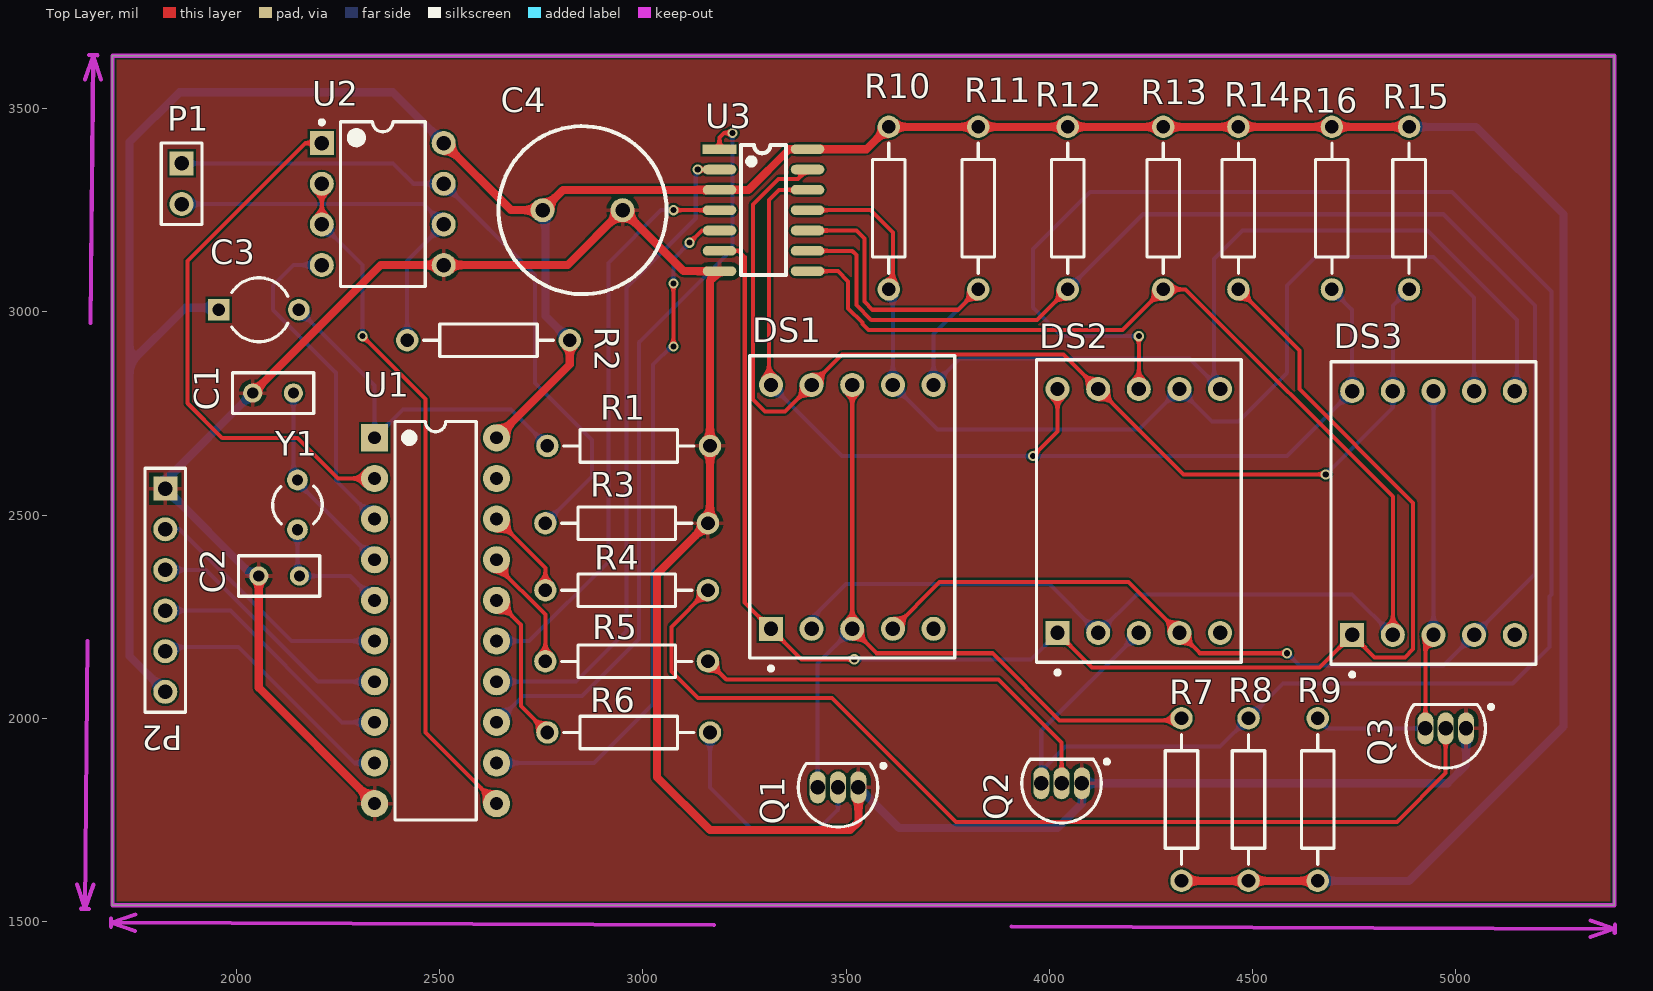
[diagram p0: Top Layer view]
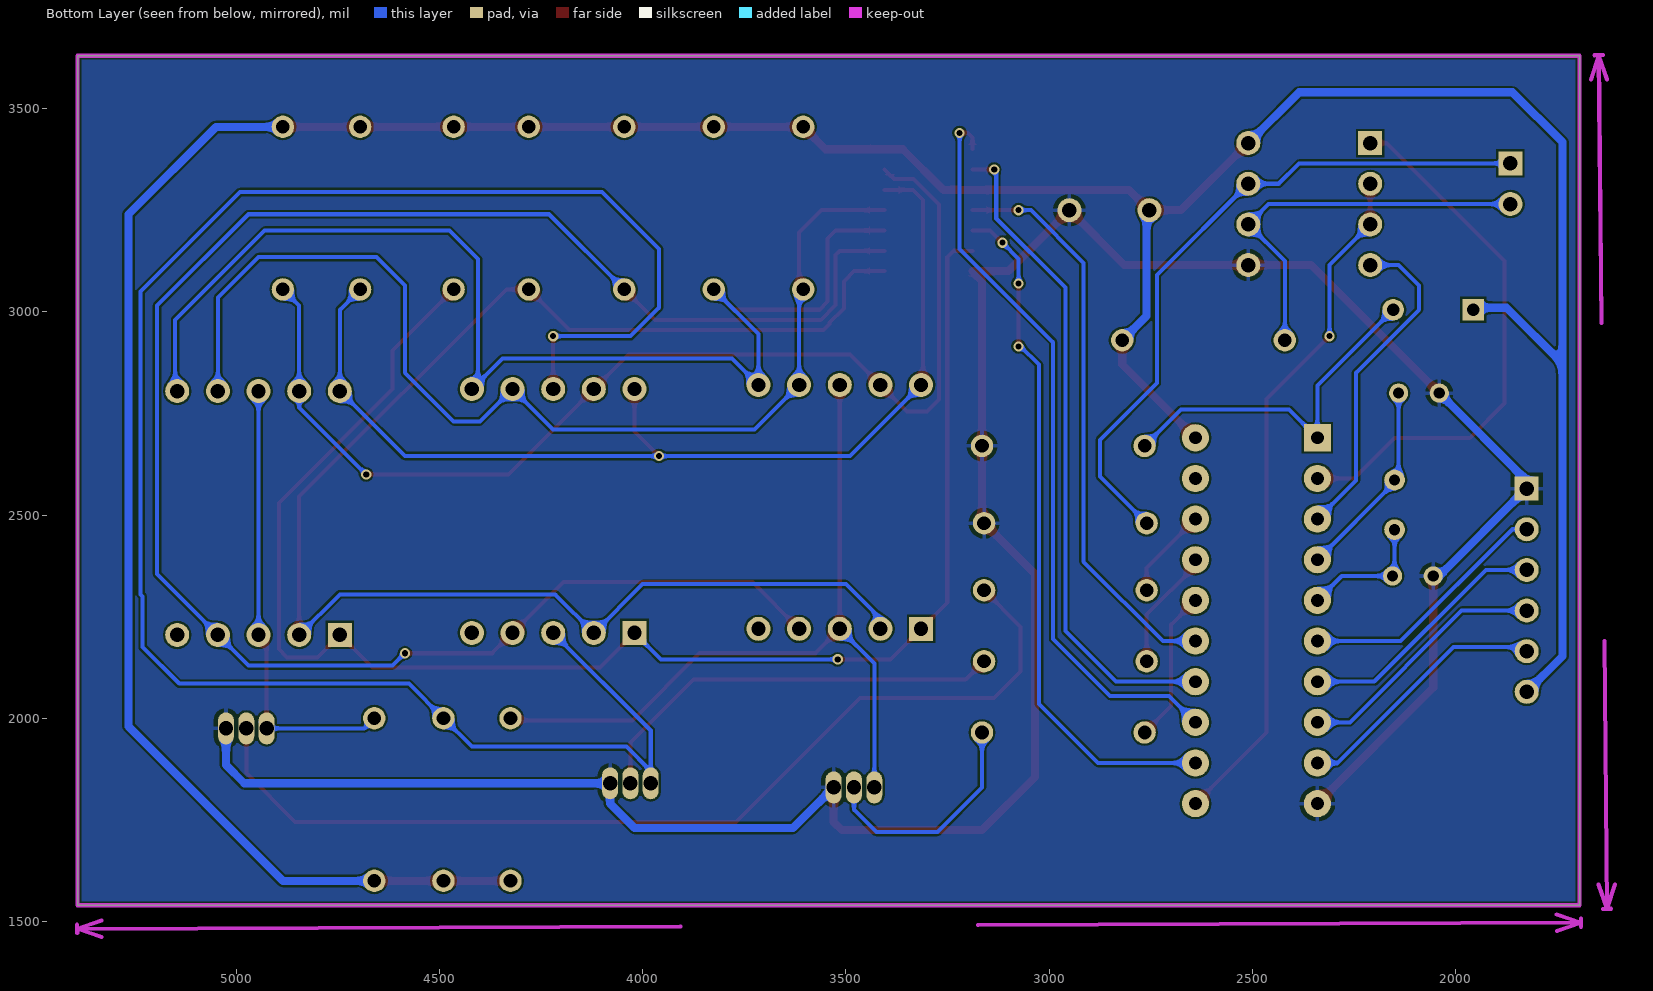
[diagram p1: Bottom Layer view, seen from below]
# Altium PCB MISC80802.PcbDoc
Units mil, origin at the board's own origin, x right, y up, seen from the top; angles counter-clockwise.
Board outline 3695 x 2090 mil, 2 copper layers (Top Layer, Bottom Layer); 32 components, 34 nets, 131 pads, 12 vias.

## Layer stack, top to bottom (the 12.6 mil dielectric is the usual default, probably not edited)
Top Solder: solder mask 0.4, Solder Resist, Dk 3.5
Top Layer: signal copper 1.4
Dielectric 1: dielectric 12.6, FR-4, Dk 4.8
Bottom Layer: signal copper 1.4
Bottom Solder: solder mask 0.4, Solder Resist, Dk 3.5

## Board outline
1695,1540 1695,3630 5390,3630 5390,1540

## Design rules (kind name [scope] priority, off if disabled: settings)
Clearance [All] p1: gap=5
MinimumSolderMaskSliver [All] p1: minsoldermaskwidth=0
PolygonConnect [All] p1: connectstyle=Relief reliefconductorwidth=10 reliefentries=4 polygonreliefangle="90 Angle" airgapwidth=10
RoutingVias [All] p1: holewidth=28 width=50 viastyle="Through Hole" minholewidth=28 minwidth=50 maxholewidth=28 maxwidth=50
SilkToSilkClearance [All] p1: silktosilkclearance=0
SilkToSolderMaskClearance [IsPad] p1: minsilkscreentomaskgap=0 clearancetoexposedcopper=TRUE
SolderMaskExpansion [All] p1: expansion=4
Width [All] p1: maxlimit=20 minlimit=10 preferedwidth=10
27 further rules are at their usual default settings.

## Components (designator, comment, footprint, x,y, rotation, side; value= is the part's Value field where it differs from the comment)
C1 "30p" RAD-0.1 2090,2800 r180 top
C2 "30p" RAD-0.1 2105,2350 r180 top
C3 "Cap Pol2" CAPR5-4X5 2055,3005 r0 top
C4 "Cap Pol2" RB5-10.5 2841.57,3255 r0 top
DS1 "Dpy Blue-CA" H 3515,2520 r0 top
DS2 "Dpy Blue-CA" H 4220,2510 r0 top
DS3 "Dpy Blue-CA" H 4945,2505 r0 top
P1 "Header 2" HDR1X2 1865,3365 r270 top
P2 "Header 6" HDR1X6 1825,2565 r270 top
Q1 "9013" TO-92A 3480,1830 r90 top
Q2 "9013" TO-92A 4030,1840 r90 top
Q3 "9013" TO-92A 4975,1975 r90 top
R1 "Res2" AXIAL-0.4 2965,2670 r180 top
R2 "Res2" AXIAL-0.4 2620,2930 r0 top
R3 "Res2" AXIAL-0.4 2960,2480 r180 top
R4 "Res2" AXIAL-0.4 2960,2315 r180 top
R5 "Res2" AXIAL-0.4 2960,2140 r180 top
R6 "Res2" AXIAL-0.4 2965,1965 r180 top
R7 "Res2" AXIAL-0.4 4325,1800 r90 top
R8 "Res2" AXIAL-0.4 4490,1800 r90 top
R9 "Res2" AXIAL-0.4 4660,1800 r90 top
R10 "Res2" AXIAL-0.4 3605,3255 r270 top
R11 "Res2" AXIAL-0.4 3825,3255 r270 top
R12 "Res2" AXIAL-0.4 4045,3255 r270 top
R13 "Res2" AXIAL-0.4 4280,3255 r270 top
R14 "Res2" AXIAL-0.4 4465,3255 r270 top
R15 "Res2" AXIAL-0.4 4885,3255 r270 top
R16 "Res2" AXIAL-0.4 4695,3255 r270 top
U1 "AT89C2051" DIP20 2490,2240 r0 top
U2 "MAX1487EPA" PA8 2360,3265 r0 top
U3 "SN74LS49D" SOP14 3188.46,3400 r0 top
Y1 "XTAL" R38 2150,2525 r0 top

## Footprints (in the part's own frame and the unit in brackets; to place one, negate y for a bottom-side part, rotate by r counter-clockwise, add the part's x,y. Pads: shape width x height; smd on the part's side, far side on the other; paste and mask are expansions set on the pad)
AXIAL-0.4 [mm] "Axial Device, Thru-Hole; 2 Leads; 0.4 in Pin Spacing"
  round 1.4 hole 0.85: 1(-5.08,0) 2(5.08,0)
  silkscreen extent -4.06,-1.02 4.06,1.02
CAPR5-4X5 [mm] "Capacitor; 2 Leads"
  rect 1.35x1.35 hole 0.8: 1(-2.5,0)
  round 1.35 hole 0.8: 2(2.5,0)
  silkscreen extent -1.69,-2 1.82,2
DIP20 [mm]
  rect 1.7x1.7 hole 0.8: 1(-3.81,11.43)
  round 1.7 hole 0.8: 2(-3.81,8.89) 3(-3.81,6.35) 4(-3.81,3.81) 5(-3.81,1.27) 6(-3.81,-1.27) 7(-3.81,-3.81) 8(-3.81,-6.35) 9(-3.81,-8.89) 10(-3.81,-11.43) 11(3.81,-11.43) 12(3.81,-8.89) 13(3.81,-6.35) 14(3.81,-3.81) 15(3.81,-1.27) 16(3.81,1.27) 17(3.81,3.81) 18(3.81,6.35) 19(3.81,8.89) 20(3.81,11.43)
  silkscreen extent -2.54,-12.45 2.54,12.45, body extent -4,-13.19 4,13.21, height 4.54
H [mm] "LED, 7-Segment Display, 14.2 mm, RHD; 10 Leads; Row Space 15.24 mm; Pitch 2.54 mm"
  rect 1.5x1.5 hole 0.9: 1(-5.08,-7.62)
  round 1.5 hole 0.9: 2(-2.54,-7.62) 3(0,-7.62) 4(2.54,-7.62) 5(5.08,-7.62) 6(5.08,7.62) 7(2.54,7.62) 8(0,7.62) 9(-2.54,7.62) 10(-5.08,7.62)
  silkscreen extent -6.4,-10.22 6.4,9.45, body extent -6.4,-9.45 6.4,9.45, height 8.25
HDR1X2 [mm] "Connector; Header; 2 Position"
  rect 1.5x1.5 hole 0.9: 1(0,0)
  round 1.5 hole 0.9: 2(2.54,0)
  silkscreen extent -1.27,-1.27 3.81,1.27
HDR1X6 [mm] "Connector; Header; 6 Position"
  rect 1.5x1.5 hole 0.9: 1(0,0)
  round 1.5 hole 0.9: 2(2.54,0) 3(5.08,0) 4(7.62,0) 5(10.16,0) 6(12.7,0)
  silkscreen extent -1.27,-1.27 13.97,1.27
PA8 [mm] "DIP, 8-Leads, Row Spacing 7.62mm, Pitch 2.54mm, Body 9.38x7.24mm"
  rect 1.5x1.5 hole 0.9: 1(-3.81,3.81)
  round 1.5 hole 0.9: 2(-3.81,1.27) 3(-3.81,-1.27) 4(-3.81,-3.81) 5(3.81,-3.81) 6(3.81,-1.27) 7(3.81,1.27) 8(3.81,3.81)
  silkscreen extent -3.93,-5.15 2.65,5.23, body extent -3.6,-5.15 3.6,5.15, height 4.58
R38 [mm] "Crystal, Thru-Hole; 2 Leads; Body 3.1 x 8.2 mm (Dia.xH)"
  round 1.3 hole 0.7: 1(0,1.55) 2(0,-1.55)
  silkscreen extent -1.55,-1.19 1.55,1.17
RAD-0.1 [mm] "Radial Cap, Thru-Hole; 2 Leads; 0.1 in Pin Spacing"
  round 1.2 hole 0.7: 1(-1.27,0) 2(1.27,0)
  silkscreen extent -2.54,-1.27 2.54,1.27
RB5-10.5 [mm] "Capacitor (Radial); 2 Leads"
  round 1.5 hole 0.9: 1(-2.246,-0.127) 2(2.754,-0.127)
  silkscreen extent -4.99,-5.38 5.5,5.12
SOP14 [mm]
  rect 2.1x0.6 smd: 1(0,0)
  oval 2.1x0.6 smd: 2(0,-1.27) 3(0,-2.54) 4(0,-3.81) 5(0,-5.08) 6(0,-6.35) 7(0,-7.62) 8(5.5,-7.62) 9(5.5,-6.35) 10(5.5,-5.08) 11(5.5,-3.81) 12(5.5,-2.54) 13(5.5,-1.27) 14(5.5,0)
  silkscreen extent 1.35,-7.87 4.15,0.25, body extent -0.25,-8.16 5.75,0.54, height 1.9
TO-92A [mm] "TO, Flat Index; 3 In-Line, Axial Leads; Body Dia. 4.5mm; Leads 0.51 x 0.48 mm (max)"
  oval 2x1 hole 0.9: 1(0,-1.27) 2(0,0) 3(0,1.27)
  silkscreen extent -2.48,-2.96 1.5,2.48, body extent -2.48,-2.5 1.5,2.5, height 6.86

## Part data
C1 C2: library part 瓷片电容
C3 C4: "Polarized Capacitor (Axial)"
DS1 DS2 DS3: "14.2 mm General Purpose Blue 7-Segment Display: CA, RH DP, Gray Surface"
P1: "Header, 2-Pin"
P2: "Header, 6-Pin"
Q1 Q2 Q3: library part 2N3904, "NPN General Purpose Amplifier"
R1 R2 R3 R4 R5 R6 R7 R8 R9 R10 R11 R12 R13 R14 R15 R16: "Resistor"
U1: library part AT89C2051-24PU
Y1: "Crystal Oscillator"

## Via types
v1: diameter 25, hole 15, Top Layer to Bottom Layer, 12 vias

## Nets (pads, with @x,y where several pads share a name; then routed paths per layer and width w, separated by ;. In a path a pad name is that pad's centre, name@x,y a point inside that pad or via, vN(x,y) a via of type N, cw(c..) or ccw(c..) an arc to the next point about the centre after c; other vN are vias at no path point)
D1: DS1.7 DS2.7 DS3.7 R10.2 U3.11 | length 2731.3
  Top Layer w10: U3.11 3560,3250 3615,3195 3615,3065 R10.2
  Bottom Layer w10: R10.2 3615,3045 DS1.7 3725,2710 4220,2710 DS2.7 4400,2730 4465,2730 4585,2850 4585,3065 4655,3135 4945,3135 5045,3035 DS3.7
D2: DS1.6 DS2.6 DS3.6 R11.2 U3.10 | length 3003
  Top Layer w10: U3.10 3525,3200 3545,3180 3545,3025 3565,3005 3775,3005 R11.2
  Bottom Layer w10: R11.2 3715,2945 DS1.6 3780,2885 4345,2885 DS2.6@4405,2825 ; DS2.6 DS2.6@4405,2825 ; DS3.6 5150,2810 5150,2980 4930,3200 4475,3200 4405,3130 DS2.6@4405,2825
D3: DS1.4 DS2.4 DS3.4 R12.2 U3.9 | length 4599.3
  Top Layer w10: U3.9 3515,3150 3525,3140 3525,3016.72 3561.72,2980 3970,2980 R12.2 ; DS1.4 3730,2335 4195,2335 DS2.4 4370,2160 v1(4585,2160)
  Bottom Layer w10: R12.2 4230,3240 4970,3240 5195,3015 5195,2355 DS3.4 4970,2130 4615,2130 v1(4585,2160)
D4: DS1.2 DS2.2 DS3.2 R13.2 U3.8 | length 3754.4
  Top Layer w10: U3.8 3480,3100 3505,3075 3505,3008.43 3540,2973.43 3540,2970 3555,2955 4180,2955 R13.2 4335,3055 4845,2545 DS3.2
  Bottom Layer w10: DS1.2 3415,2245 3500,2330 4000,2330 DS2.2 4215,2305 4745,2305 DS3.2
D5: DS1.1 DS2.1 DS3.1 R14.2 U3.6 | length 3810.5
  Top Layer w10: U3.6 3235.47,3150 3250.47,3135 3250.47,2284.53 DS1.1 3390,2145 v1(3520,2145) ; DS2.1 4105,2125 4665,2125 DS3.1 4800,2150 4875,2150 4895,2170 4895,2530 4615,2810 4615,2905 R14.2
  Bottom Layer w10: v1(3520,2145) 3955,2145 DS2.1
D6: DS1.9 DS2.9 DS3.9 R15.2 U3.13 | length 2791.3
  Top Layer w10: U3.13 3381.81,3326.81 3333.53,3326.81 3270.47,3263.76 3270.47,2784.53 3300,2755 3350,2755 DS1.9 3490,2895 4035,2895 DS2.9 4330,2600 v1(4680,2600)
  Bottom Layer w10: v1(4680,2600) 4845,2765 DS3.9 4845,3015 R15.2
D7: DS1.10 DS2.10 DS3.10 R16.2 U3.12 | length 2591.8
  Top Layer w10: DS1.10 3310,2825 3310,3275 3335,3300 U3.12 ; v1(3960,2645) 4020,2705 DS2.10
  Bottom Layer w10: DS1.10 3490,2645 v1(3960,2645) 4585,2645 DS3.10 4745,3005 R16.2
GND: C1.2 C2.2 C4.2 P2.1 Q1.1 Q2.1 Q3.1 R1.1 R3.1 U1.10 U2.5 U3.7 | length 6388.8
  Top Layer w20: C1.2 2355,3115 U2.5 2815,3115 C4.2 3100,3100 U3.7 3165,3076.54 R1.1 3165,2485 R3.1 3035,2355 3035,1855 3165,1725 3510,1725 3530,1745 Q1.1 ; C2.2 2055,2075 U1.10
  Bottom Layer w20: C1.2 1825,2585 P2.1 2040,2350 C2.2 ; Q1.1 3630,1730 4020,1730 4080,1790 Q2.1 4980,1840 5025,1885 Q3.1
NetC1_1: C1.1 U1.4 Y1.1 | length 492.8
  Bottom Layer w10: C1.1 2140,2596.02 Y1.1 2150,2580 U1.4
NetC2_1: C2.1 U1.5 Y1.2 | length 325.9
  Bottom Layer w10: Y1.2 2150,2355 C2.1 2280,2350 U1.5
NetC3_2: C3.2 R1.2 U1.1 | length 883.6
  Bottom Layer w10: C3.2 2340,2818.43 U1.1 2410,2760 2675,2760 R1.2
NetDS1_3: DS1.3 DS1.8 Q1.3 R7.2 | length 1930.5
  Top Layer w10: DS1.8 DS1.3 3575,2160 3860,2160 4025,1995 4320,1995 R7.2
  Bottom Layer w10: Q1.3 3430,2135 DS1.3
NetDS2_3: DS2.3 DS2.8 Q2.3 R8.2 | length 4721.3
  Top Layer w10: DS2.8 v1(4220,2940)
  Bottom Layer w10: Q2.3 Q2.3@3980,1870 ; DS2.3 3980,1970 Q2.3@3980,1870 ; v1(4220,2940) 4030,2940 3960,3010 3960,3155 4100,3295 4990,3295 5235,3050 5235,2305 5230,2300 5230,2175 5140,2085 4575,2085 R8.2 4420,1930 4040,1930 Q2.3@3980,1870
NetDS3_3: DS3.3 DS3.8 Q3.3 R9.2 | length 1141.9
  Top Layer w10: Q3.3 4925,2185 DS3.3
  Bottom Layer w10: R9.2 4685,1975 Q3.3 Q3.3@4940.31,1990.32 ; DS3.3@4940.31,2200.32 DS3.3 DS3.8
NetP1_1: P1.1 R3.2 U2.7 | length 1699.5
  Bottom Layer w10: P1.1 2385,3365 2435,3315 U2.7 2735,3090 2735,2825 2875,2685 2875,2595 R3.2
NetP1_2: P1.2 R2.1 U2.6 | length 988
  Bottom Layer w10: P1.2 2460,3265 U2.6 2420,3125 R2.1
NetP2_2: P2.2 U1.6 | length 628.9
  Bottom Layer w10: P2.2 1860,2465 2135,2190 U1.6
NetP2_3: P2.3 U1.7 | length 628.9
  Bottom Layer w10: P2.3 1925,2365 2200,2090 U1.7
NetP2_4: P2.4 U1.8 | length 628.9
  Bottom Layer w10: P2.4 1985,2265 2260,1990 U1.8
NetP2_5: P2.5 U1.9 | length 637.2
  Bottom Layer w10: P2.5 1835,2175 2005,2175 2290,1890 U1.9
NetQ1_2: Q1.2 R6.1 | length 573.3
  Bottom Layer w10: R6.1 3165,1830 3275,1720 3425,1720 3480,1775 Q1.2
NetQ2_2: Q2.2 R5.1 | length 1052.8
  Top Layer w10: R5.1 3205,2095 3875,2095 4030,1940 Q2.2
NetQ3_2: Q3.2 R4.1 | length 2455.2
  Top Layer w10: R4.1 3070,2225 3070,2115 3135,2050 3465,2050 3770,1745 4855,1745 4975,1865 Q3.2
NetR4_2: R4.2 U1.18 | length 224.7
  Top Layer w10: U1.18 2760,2370 R4.2
NetR5_2: R5.2 U1.17 | length 299.7
  Top Layer w10: U1.17 2640,2374.81 2760,2254.81 R5.2
NetR6_2: R6.2 U1.16 | length 376.8
  Top Layer w10: U1.16 2700,2230 2700,2030 R6.2
NetU1_2: U1.2 U2.1 | length 1336.8
  Top Layer w10: U2.1 2170,3415 1880,3125 1880,2775 1965,2690 2150,2690 2250,2590 U1.2
NetU1_3: U1.3 U2.4 | length 819.3
  Bottom Layer w10: U2.4 2140,3115 2090,3065 2090,3005 2245,2850 2245,2585 U1.3
NetU1_11: U1.11 U2.2 U2.3 | length 1703.1
  Top Layer w10: U2.3 U2.2 ; v1(2310,2940) 2465,2785 2465,1965 U1.11
  Bottom Layer w10: U2.3 2310,3115 v1(2310,2940)
NetU1_12: U1.12 U3.5 | length 1701.2
  Top Layer w10: v1(3075,2915) v1(3075,3070) ; v1(3115,3170) 3145,3200 U3.5
  Bottom Layer w10: U1.12 2880,1890 3025,2035 3025,2870 v1@3070,2915 ; v1(3075,3070) 3075,3130 v1(3115,3170)
NetU1_13: U1.13 U3.1 | length 1840
  Top Layer w10: U3.1 3188.46,3428.46 3200,3440 v1(3220,3440)
  Bottom Layer w10: U1.13 2705,2055 2850,2055 2990,2195 2990,2925 3220,3155 v1(3220,3440)
NetU1_14: U1.14 U3.2 | length 1632.7
  Top Layer w10: v1(3135,3350) U3.2
  Bottom Layer w10: U1.14 2835,2090 2960,2215 2960,3060 3130,3230 3130,3345 v1(3135,3350)
NetU1_15: U1.15 U3.4 | length 1418.1
  Top Layer w10: v1(3075,3250) U3.4
  Bottom Layer w10: U1.15 2720,2190 2915,2385 2915,3120 3045,3250 v1(3075,3250)
VCC: C3.1 C4.1 P2.6 R2.2 R7.1 R8.1 R9.1 R10.1 R11.1 R12.1 R13.1 R14.1 R15.1 R16.1 U1.20 U2.8 U3.3 U3.14 | length 8559.2
  Top Layer w20: U2.8 2675,3250 C4.1 2803.15,3300 U3.3 3260,3300 3360,3400 U3.14 3550,3400 R10.1 R11.1 R12.1 R13.1 R14.1 R16.1 R15.1 ; U1.20 2820,2870 R2.2 ; R7.1 R8.1 R9.1
  Bottom Layer w20: P2.6 1737.33,2152.67 1737.33,2872.33 ; C3.1 1951.58,3010 1875,3010 1737.33,2872.33 ; U2.8 2385,3540 1860,3540 1737.33,3417.33 1737.33,2872.33 ; C4.1 2760,3243.15 2760,2990 R2.2 ; R9.1 4885,1600 5265,1980 5265,3240 5050,3455 R15.1
pads on no net: DS1.5 DS2.5 DS3.5 U1.19

## Polygon pours and split planes (outlines as drawn)
GND on Bottom Layer "Top Layer-No Net" (solid, remove dead copper, pour order 4): 1525,3815 5575,3815 5590,3800 5520,3730 5520,1350 1530,1350 1500,1380
GND on Top Layer "Top Layer-No Net" (solid, remove dead copper, pour order 6): 1205,3915 5570,3915 5635,3850 5690,3795 5690,1020 1335,1020 1015,1340

## Keep-outs
Keep-Out Layer:
  lines w10: 1608.2,1591.39 1627.63,1531.2 ; 1617.63,1531.3 1637.63,1531.11 ; 1627.09,3571.4 1647.67,3631.2 ; 1633.92,2190.34 1627.63,1531.2 ; 1637.67,3631.3 1657.67,3631.11 ; 1641.38,2972.07 1647.67,3631.2 ; 1648.2,1591.01 1627.63,1531.2 ; 1667.09,3571.02 1647.67,3631.2 ; 1690.99,1487.05 1691.07,1507.05 ; 1750.95,1476.8 1691.03,1497.05 ; 1751.11,1516.8 1691.03,1497.05 ; 3175.15,1491.03 1691.03,1497.05 ; 3906.91,1488.06 5391.03,1482.05 ; 5330.95,1462.29 5391.03,1482.05 ; 5331.11,1502.29 5391.03,1482.05 ; 5390.99,1472.05 5391.07,1492.05 ; 1695,1540 1695,3630 5390,3630 5390,1600 5390,1540 1695,1540
  text "2100.095 (mil)" at 1670,2200 h60 r89.45
  text "3700.03 (mil)" at 3185,1455 h60 r359.77